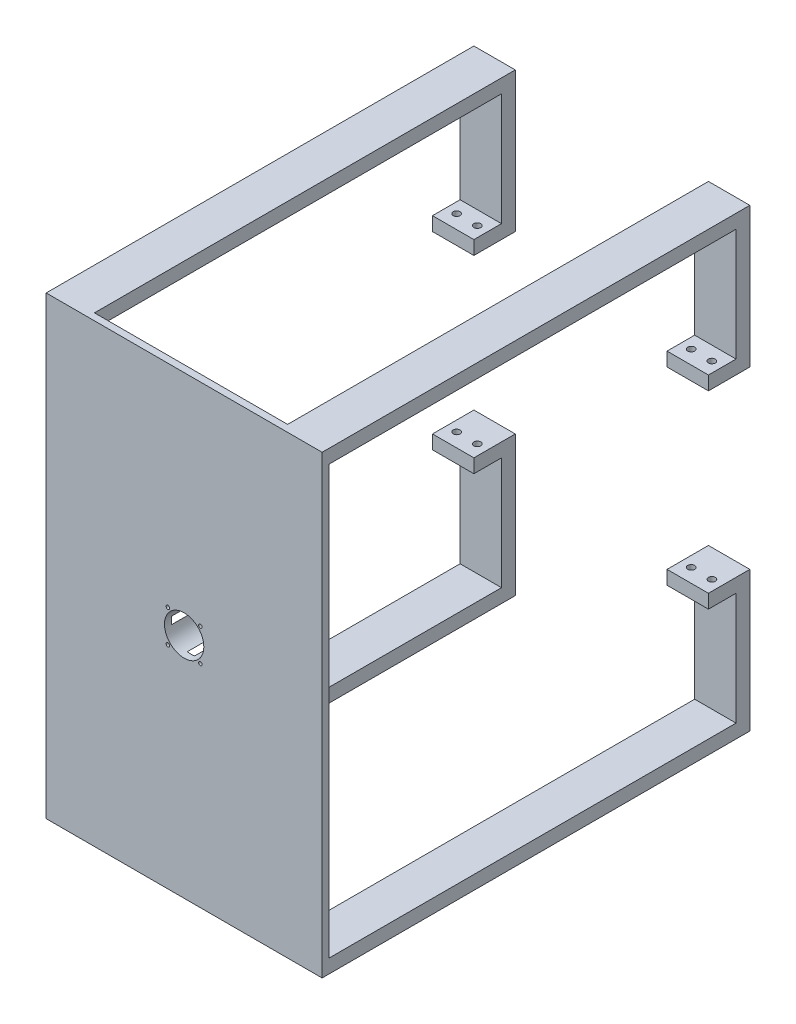
from build123d import *
from build123d.topology import SkipClean

# Parameters (mm, degrees)
SKETCH_1_W                                 = 400
SKETCH_1_H                                 = 660
SKETCH_1_R                                 = 28.5
EXTRUDE_1_DEPTH                            = 10
EXTRUDE_START                              = 62.5
EXTRUDE_3_DEPTH                            = 62.5
SKETCH_4_W                                 = 60
SKETCH_4_H                                 = 620
EXTRUDE_4_DEPTH                            = 20
SKETCH_5_W                                 = 60
SKETCH_5_H                                 = 20
EXTRUDE_5_DEPTH                            = 203
MIRROR_3_COPY_1_SKETCH_W                   = 60
MIRROR_3_COPY_1_SKETCH_H                   = 20
MIRROR_3_COPY_1_DEPTH                      = 203
MIRROR_3_AT_THE_SECOND_PLANE_COPY_1_SKET_W = 60
MIRROR_3_AT_THE_SECOND_PLANE_COPY_1_SKET_H = 20
MIRROR_3_AT_THE_SECOND_PLANE_COPY_1_DEPTH  = 203
MIRROR_3_AT_THE_SECOND_PLANE_COPY_2_SKET_W = 60
MIRROR_3_AT_THE_SECOND_PLANE_COPY_2_SKET_H = 20
MIRROR_3_AT_THE_SECOND_PLANE_COPY_2_DEPTH  = 203
MIRROR_3_AT_THE_SECOND_PLANE_COPY_3_SKET_W = 60
MIRROR_3_AT_THE_SECOND_PLANE_COPY_3_SKET_H = 20
MIRROR_3_AT_THE_SECOND_PLANE_COPY_3_DEPTH  = 203
SKETCH_6_W                                 = 60
SKETCH_6_H                                 = 60
EXTRUDE_6_DEPTH                            = 20
MIRROR_5_COPY_1_SKETCH_W                   = 60
MIRROR_5_COPY_1_SKETCH_H                   = 60
MIRROR_5_COPY_1_DEPTH                      = 20
CUT_EXTRUDE_1_REACH                        = 1169.96
SKETCH_7_R                                 = 5
SKETCH_8_R                                 = 2.6
CUT_EXTRUDE_2_DEPTH                        = 1172.641719812


with BuildPart() as part:
    # 草图1 → 凸台-拉伸1 (new body)
    with BuildSketch(Plane.XY):
        with Locations((674.357789758, 143.120254367)):
            Rectangle(SKETCH_1_W, SKETCH_1_H)
        with Locations((674.357789758, 143.120254367)):
            Circle(SKETCH_1_R, mode=Mode.SUBTRACT)
    extrude(amount=EXTRUDE_1_DEPTH)

    # 草图3 → 凸台-拉伸3 (add)
    with SkipClean():  # the faces are left unmerged after this step: merging them gives an invalid solid
        with BuildSketch(Plane(origin=(0, 0, 0), x_dir=(-1, 0, 0), z_dir=(0, 0, -1)).offset(EXTRUDE_START)):
            with BuildLine():
                Line((-702.357789758, 148.435327273), (-702.357789758, 166.620254367))
                ThreePointArc((-702.357789758, 166.620254367), (-701.039770274, 169.802234882), (-697.857789758, 171.120254367))
                Line((-697.857789758, 171.120254367), (-679.672862665, 171.120254367))
                ThreePointArc((-679.672862665, 171.120254367), (-694.510333022, 163.27279763), (-702.357789758, 148.435327273))
            make_face()
            with BuildLine():
                Line((-679.672862665, 115.120254367), (-697.857789758, 115.120254367))
                ThreePointArc((-697.857789758, 115.120254367), (-701.039770274, 116.438273851), (-702.357789758, 119.620254367))
                Line((-702.357789758, 119.620254367), (-702.357789758, 137.80518146))
                ThreePointArc((-702.357789758, 137.80518146), (-694.510333022, 122.967711103), (-679.672862665, 115.120254367))
            make_face()
            with BuildLine():
                Line((-646.357789758, 137.80518146), (-646.357789758, 119.620254367))
                ThreePointArc((-646.357789758, 119.620254367), (-647.675809243, 116.438273851), (-650.857789758, 115.120254367))
                Line((-650.857789758, 115.120254367), (-669.042716852, 115.120254367))
                ThreePointArc((-669.042716852, 115.120254367), (-654.205246495, 122.967711103), (-646.357789758, 137.80518146))
            make_face()
            with BuildLine():
                Line((-669.042716852, 171.120254367), (-650.857789758, 171.120254367))
                ThreePointArc((-650.857789758, 171.120254367), (-647.675809243, 169.802234882), (-646.357789758, 166.620254367))
                Line((-646.357789758, 166.620254367), (-646.357789758, 148.435327273))
                ThreePointArc((-646.357789758, 148.435327273), (-654.205246495, 163.27279763), (-669.042716852, 171.120254367))
            make_face()
        extrude(amount=-EXTRUDE_3_DEPTH)

    # 草图4 → 凸台-拉伸4 (add)
    with SkipClean():  # the faces are left unmerged after this step: merging them gives an invalid solid
        with BuildSketch(Plane.XZ.offset(186.879745633)):
            with Locations((504.357789758, -300)):
                Rectangle(SKETCH_4_W, SKETCH_4_H)
            with Locations((844.357789758, -300)):
                Rectangle(SKETCH_4_W, SKETCH_4_H)
        extrude_4 = extrude(amount=-EXTRUDE_4_DEPTH)

    # 镜向1: 凸台-拉伸4 across plane
    with SkipClean():  # the faces are left unmerged after this step: merging them gives an invalid solid
        add(extrude_4.mirror(Plane(origin=(0, 143.120254367, 0), x_dir=(0, 0, 1), z_dir=(0, -1, 0))))

    # 草图5 → 凸台-拉伸5 (add)
    with SkipClean():  # the faces are left unmerged after this step: merging them gives an invalid solid
        with BuildSketch(Plane(origin=(0, 473.120254367, 0), x_dir=(1, 0, 0), z_dir=(0, 1, 0))):
            with Locations((844.357789758, 600)):
                Rectangle(SKETCH_5_W, SKETCH_5_H)
        extrude_5 = extrude(amount=-EXTRUDE_5_DEPTH)

    # 镜向2: 凸台-拉伸5 across plane
    with SkipClean():  # the faces are left unmerged after this step: merging them gives an invalid solid
        add(extrude_5.mirror(Plane(origin=(674.357789758, 0, 0), x_dir=(0, 0, 1), z_dir=(1, 0, 0))))

    # 镜向3: 凸台-拉伸5 across plane
    with SkipClean():  # the faces are left unmerged after this step: merging them gives an invalid solid
        add(extrude_5.mirror(Plane(origin=(0, 143.120254367, 0), x_dir=(0, 0, 1), z_dir=(0, -1, 0))))

    # 镜向3 copy 1 sketch → 镜向3 copy 1 (add)
    with SkipClean():  # the faces are left unmerged after this step: merging them gives an invalid solid
        with BuildSketch(Plane(origin=(1348.715579517, -186.879745633, 0), x_dir=(-1, 0, 0), z_dir=(0, -1, 0))):
            with Locations((844.357789758, 600)):
                Rectangle(MIRROR_3_COPY_1_SKETCH_W, MIRROR_3_COPY_1_SKETCH_H)
        extrude(amount=-MIRROR_3_COPY_1_DEPTH)

    # 镜向3 at the second plane: 凸台-拉伸5 across plane
    with SkipClean():  # the faces are left unmerged after this step: merging them gives an invalid solid
        add(extrude_5.mirror(Plane(origin=(674.357789758, 0, 0), x_dir=(0, 0, 1), z_dir=(1, 0, 0))))

    # 镜向3 at the second plane copy 1 sket → 镜向3 at the second plane copy 1 (add)
    with SkipClean():  # the faces are left unmerged after this step: merging them gives an invalid solid
        with BuildSketch(Plane(origin=(0, 473.120254367, 0), x_dir=(1, 0, 0), z_dir=(0, 1, 0))):
            with Locations((844.357789758, 600)):
                Rectangle(MIRROR_3_AT_THE_SECOND_PLANE_COPY_1_SKET_W, MIRROR_3_AT_THE_SECOND_PLANE_COPY_1_SKET_H)
        extrude(amount=-MIRROR_3_AT_THE_SECOND_PLANE_COPY_1_DEPTH)

    # 镜向3 at the second plane copy 2 sket → 镜向3 at the second plane copy 2 (add)
    with SkipClean():  # the faces are left unmerged after this step: merging them gives an invalid solid
        with BuildSketch(Plane(origin=(1348.715579517, -186.879745633, 0), x_dir=(-1, 0, 0), z_dir=(0, -1, 0))):
            with Locations((844.357789758, 600)):
                Rectangle(MIRROR_3_AT_THE_SECOND_PLANE_COPY_2_SKET_W, MIRROR_3_AT_THE_SECOND_PLANE_COPY_2_SKET_H)
        extrude(amount=-MIRROR_3_AT_THE_SECOND_PLANE_COPY_2_DEPTH)

    # 镜向3 at the second plane copy 3 sket → 镜向3 at the second plane copy 3 (add)
    with SkipClean():  # the faces are left unmerged after this step: merging them gives an invalid solid
        with BuildSketch(Plane.XZ.offset(186.879745633)):
            with Locations((844.357789758, -600)):
                Rectangle(MIRROR_3_AT_THE_SECOND_PLANE_COPY_3_SKET_W, MIRROR_3_AT_THE_SECOND_PLANE_COPY_3_SKET_H)
        extrude(amount=-MIRROR_3_AT_THE_SECOND_PLANE_COPY_3_DEPTH)

    # 草图6 → 凸台-拉伸6 (add)
    with SkipClean():  # the faces are left unmerged after this step: merging them gives an invalid solid
        with BuildSketch(Plane.XZ.offset(-270.120254367)):
            with Locations((844.357789758, -580)):
                Rectangle(SKETCH_6_W, SKETCH_6_H)
        extrude_6 = extrude(amount=-EXTRUDE_6_DEPTH)

    # 镜向4: 凸台-拉伸6 across plane
    with SkipClean():  # the faces are left unmerged after this step: merging them gives an invalid solid
        add(extrude_6.mirror(Plane(origin=(674.357789758, 0, 0), x_dir=(0, 0, 1), z_dir=(1, 0, 0))))

    # 镜向5: 凸台-拉伸6 across plane
    with SkipClean():  # the faces are left unmerged after this step: merging them gives an invalid solid
        add(extrude_6.mirror(Plane(origin=(0, 143.120254367, 0), x_dir=(0, 0, 1), z_dir=(0, -1, 0))))

    # 镜向5 copy 1 sketch → 镜向5 copy 1 (add)
    with SkipClean():  # the faces are left unmerged after this step: merging them gives an invalid solid
        with BuildSketch(Plane(origin=(1348.715579517, 16.120254367, 0), x_dir=(-1, 0, 0), z_dir=(0, 1, 0))):
            with Locations((844.357789758, -580)):
                Rectangle(MIRROR_5_COPY_1_SKETCH_W, MIRROR_5_COPY_1_SKETCH_H)
        extrude(amount=-MIRROR_5_COPY_1_DEPTH)

    # 切除-拉伸1: up to this face of the body (flat: up to its plane)
    cut_extrude_1_end = Plane(part.part.faces().sort_by_distance((844.357789758, -3.879745633, -570))[0])
    # 草图7 → 切除-拉伸1 (cut, up to the picked face)
    with BuildSketch(Plane(origin=(0, 290.120254367, 0), x_dir=(1, 0, 0), z_dir=(0, 1, 0)), mode=Mode.PRIVATE) as cut_extrude_1_sk1:
        with Locations(Location((859.357789758, 570, 0), (0, 0, 180))):
            Circle(SKETCH_7_R)
    cut_extrude_1_tool1 = split(extrude(cut_extrude_1_sk1.sketch, amount=-CUT_EXTRUDE_1_REACH, mode=Mode.PRIVATE), bisect_by=cut_extrude_1_end, keep=Keep.BOTH, mode=Mode.PRIVATE)
    # 草图7 → 切除-拉伸1 (cut, up to the picked face)
    with BuildSketch(Plane(origin=(0, 290.120254367, 0), x_dir=(1, 0, 0), z_dir=(0, 1, 0)), mode=Mode.PRIVATE) as cut_extrude_1_sk2:
        with Locations(Location((829.357789758, 570, 0), (0, 0, 180))):
            Circle(SKETCH_7_R)
    cut_extrude_1_tool2 = split(extrude(cut_extrude_1_sk2.sketch, amount=-CUT_EXTRUDE_1_REACH, mode=Mode.PRIVATE), bisect_by=cut_extrude_1_end, keep=Keep.BOTH, mode=Mode.PRIVATE)
    cut_extrude_1_1 = cut_extrude_1_tool1.solids().sort_by(Axis((859.35779, 290.120254, -570), (0, -1, 0)))[0]
    add(cut_extrude_1_1, mode=Mode.SUBTRACT)
    cut_extrude_1_2 = cut_extrude_1_tool2.solids().sort_by(Axis((829.35779, 290.120254, -570), (0, -1, 0)))[0]
    add(cut_extrude_1_2, mode=Mode.SUBTRACT)
    cut_extrude_1 = cut_extrude_1_1 + cut_extrude_1_2  # 切除-拉伸1 as one shape, for the pattern or mirror that repeats it

    # 镜向6: 切除-拉伸1 across plane
    with SkipClean():  # the faces are left unmerged after this step: merging them gives an invalid solid
        add(cut_extrude_1.mirror(Plane(origin=(674.357789758, 0, 0), x_dir=(0, 0, 1), z_dir=(1, 0, 0))), mode=Mode.SUBTRACT)

    # 草图8 → 切除-拉伸2 (cut, through all)
    with SkipClean():  # the faces are left unmerged after this step: merging them gives an invalid solid
        with BuildSketch(Plane.XY.offset(10)):
            with Locations((650.812789758, 166.665254367)):
                Circle(SKETCH_8_R)
            with Locations((650.812789758, 119.575254367)):
                Circle(SKETCH_8_R)
            with Locations((697.902789758, 119.575254367)):
                Circle(SKETCH_8_R)
            with Locations((697.902789758, 166.665254367)):
                Circle(SKETCH_8_R)
        extrude(amount=-CUT_EXTRUDE_2_DEPTH, mode=Mode.SUBTRACT)


solid = part.part
